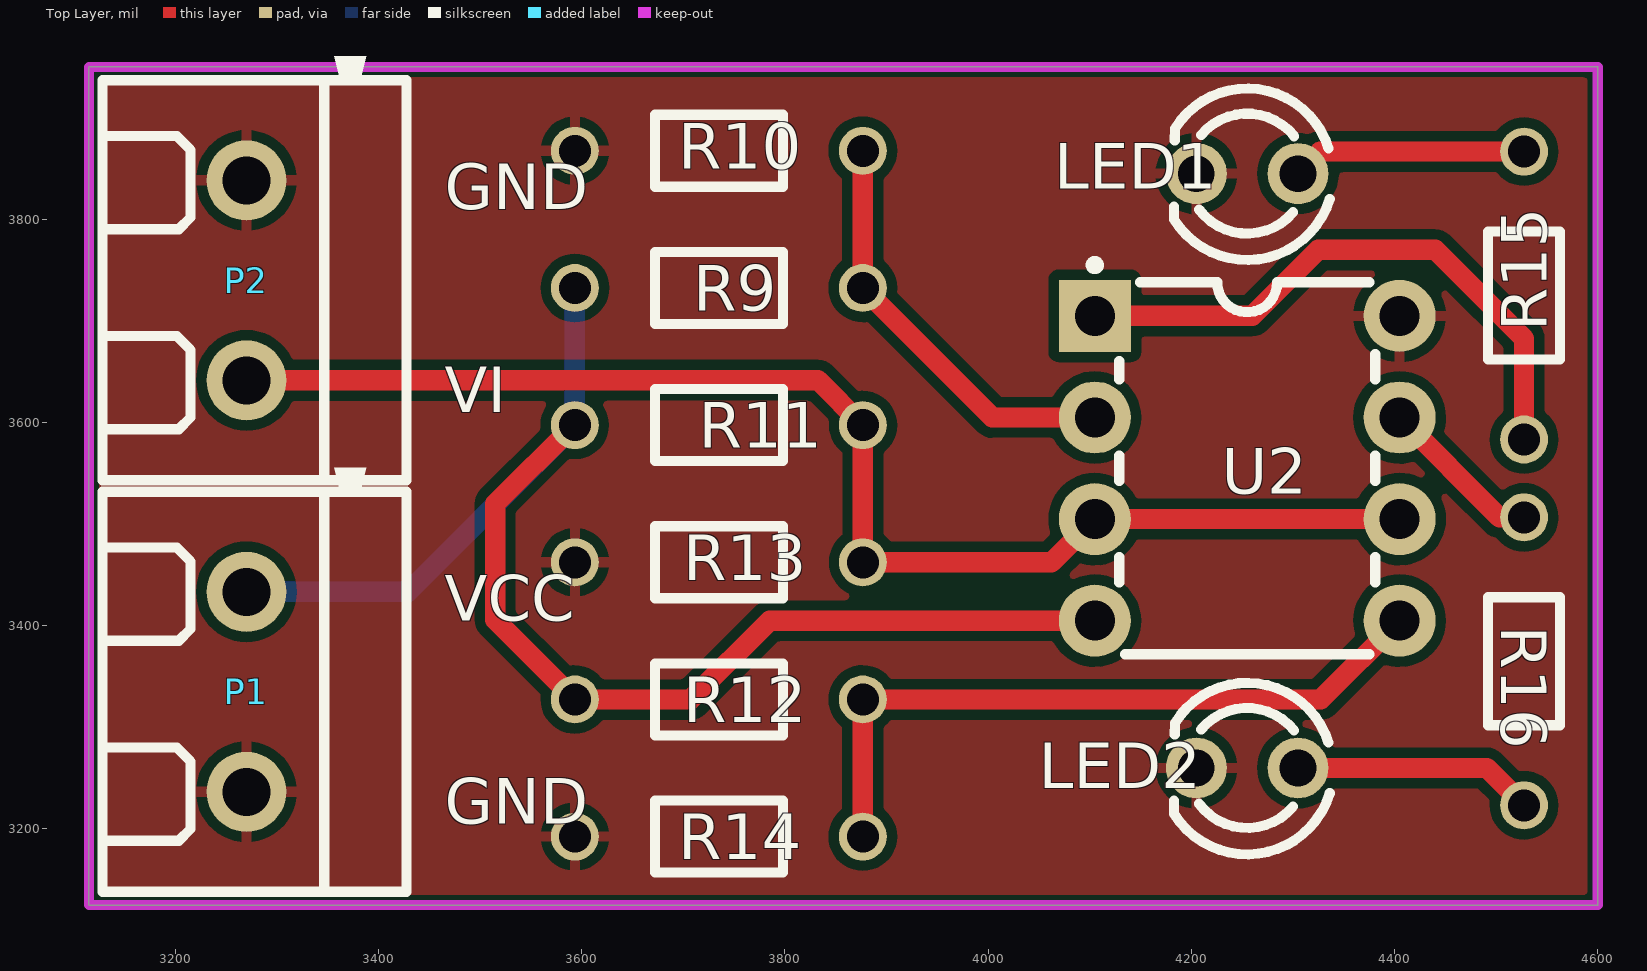
[diagram p0: Top Layer view]
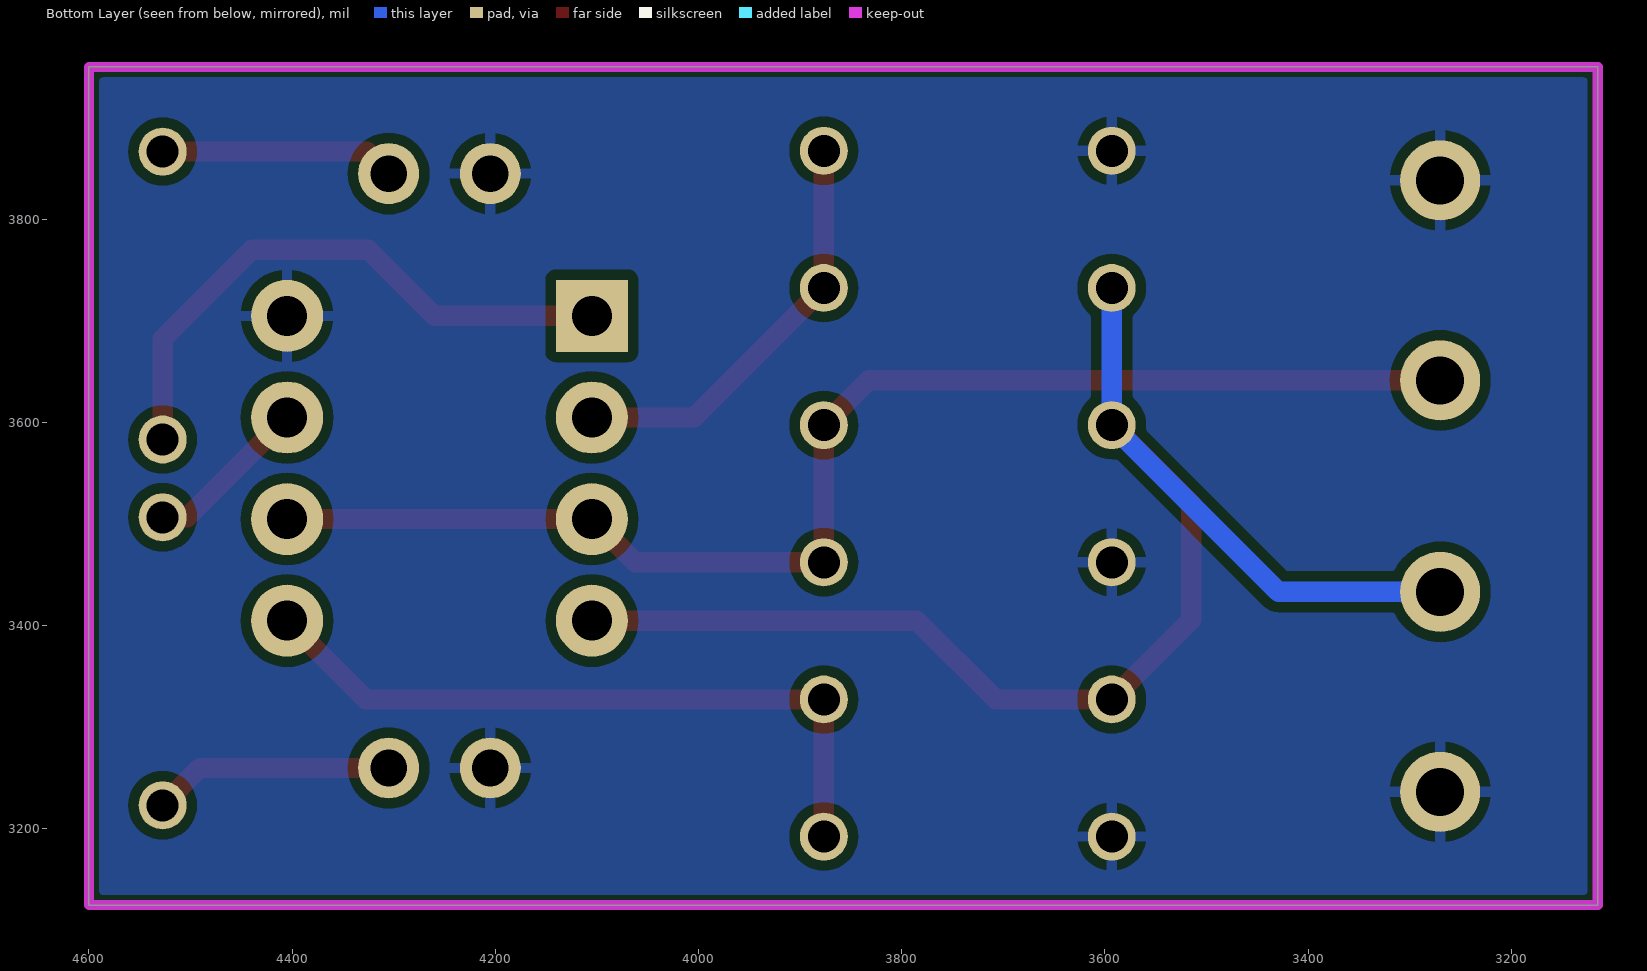
[diagram p1: Bottom Layer view, seen from below]
# Altium PCB MISC51032.pcbdoc
Units mil, origin at the board's own origin, x right, y up, seen from the top; angles counter-clockwise.
Board outline 1485 x 825 mil, 2 copper layers (Top Layer, Bottom Layer), stack 62.206 mil thick; 13 components, 9 nets, 32 pads, 0 vias.

## Layer stack, top to bottom
Top Solder Mask Layer: solder mask 0.394, Dk 3.3
Top Layer: signal copper 1.379
Dielectric1: surface 59.449, FR4, Dk 4.5
Bottom Layer: signal copper 1.378
Bottom Solder Mask Layer: solder mask 0.394, Dk 3.3

## Board outline
3115,3950 3115,3125 4600,3125 4600,3950

## Design rules (kind name [scope] priority, off if disabled: settings)
BoardOutlineClearance copperThickness2oz_1 [All] p2 off: genericclearance=7.99 ignorepadtopadclearanceinfootprint=FALSE except(0: Arc-SplitContinuation Track-SplitContinuation SMDPad-SplitContinuation THPad-SplitContinuation Via-SplitContinuation Fill-SplitContinuation Region-SplitContinuation Poly-SplitContinuation Text-SplitContinuation Hole-SplitContinuation; 5.98: Arc-CutoutEdge Track-CutoutEdge SMDPad-CutoutEdge THPad-CutoutEdge Via-CutoutEdge Text-CutoutEdge; 6.9: Hole-OutlineEdge Hole-CutoutEdge; 10: Poly-OutlineEdge Poly-CutoutEdge; 11.81: Arc-OutlineEdge Track-OutlineEdge SMDPad-OutlineEdge THPad-OutlineEdge Via-OutlineEdge Fill-OutlineEdge Region-OutlineEdge Text-OutlineEdge Fill-CutoutEdge Region-CutoutEdge)
BoardOutlineClearance Plane_innerPlane_1 [All] p4 off: genericclearance=4.02 ignorepadtopadclearanceinfootprint=FALSE except(0: Arc-SplitContinuation Track-SplitContinuation SMDPad-SplitContinuation THPad-SplitContinuation Via-SplitContinuation Fill-SplitContinuation Region-SplitContinuation Poly-SplitContinuation Text-SplitContinuation Hole-SplitContinuation; 5.98: Arc-CutoutEdge Track-CutoutEdge SMDPad-CutoutEdge THPad-CutoutEdge Via-CutoutEdge Text-CutoutEdge; 6.9: Hole-OutlineEdge Hole-CutoutEdge; 10: Poly-OutlineEdge Poly-CutoutEdge; 11.81: Arc-OutlineEdge Track-OutlineEdge SMDPad-OutlineEdge THPad-OutlineEdge Via-OutlineEdge Fill-OutlineEdge Region-OutlineEdge Text-OutlineEdge Fill-CutoutEdge Region-CutoutEdge)
BoardOutlineClearance Copper_copperRegion_1 [All] p6 off: genericclearance=4.02 ignorepadtopadclearanceinfootprint=FALSE except(0: Arc-SplitContinuation Track-SplitContinuation SMDPad-SplitContinuation THPad-SplitContinuation Via-SplitContinuation Fill-SplitContinuation Region-SplitContinuation Poly-SplitContinuation Text-SplitContinuation Hole-SplitContinuation; 5.98: Arc-CutoutEdge Track-CutoutEdge SMDPad-CutoutEdge THPad-CutoutEdge Via-CutoutEdge Text-CutoutEdge; 6.9: Hole-OutlineEdge Hole-CutoutEdge; 10: Poly-OutlineEdge Poly-CutoutEdge; 11.81: Arc-OutlineEdge Track-OutlineEdge SMDPad-OutlineEdge THPad-OutlineEdge Via-OutlineEdge Fill-OutlineEdge Region-OutlineEdge Text-OutlineEdge Fill-CutoutEdge Region-CutoutEdge)
BoardOutlineClearance copperThickness1oz_1 [All] p8: genericclearance=4.02 ignorepadtopadclearanceinfootprint=FALSE except(0: Arc-SplitContinuation Track-SplitContinuation SMDPad-SplitContinuation THPad-SplitContinuation Via-SplitContinuation Fill-SplitContinuation Region-SplitContinuation Poly-SplitContinuation Text-SplitContinuation Hole-SplitContinuation; 5.98: Arc-CutoutEdge Track-CutoutEdge SMDPad-CutoutEdge THPad-CutoutEdge Via-CutoutEdge Text-CutoutEdge; 6.9: Hole-OutlineEdge Hole-CutoutEdge; 10: Poly-OutlineEdge Poly-CutoutEdge; 11.81: Arc-OutlineEdge Track-OutlineEdge SMDPad-OutlineEdge THPad-OutlineEdge Via-OutlineEdge Fill-OutlineEdge Region-OutlineEdge Text-OutlineEdge Fill-CutoutEdge Region-CutoutEdge)
Clearance copperThickness2oz [All] p1 off: gap=7.99 ignorepadtopadclearanceinfootprint=FALSE except(5.98: SMDPad-Track SMDPad-SMDPad THPad-Track SMDPad-THPad THPad-THPad Track-Via SMDPad-Via THPad-Via Via-Via Fill-SMDPad Region-SMDPad Fill-THPad Region-THPad Fill-Via Region-Via Fill-Fill Fill-Region Region-Region Arc-Track Arc-SMDPad Arc-THPad Arc-Via Fill-Arc Region-Arc Arc-Arc Text-Track SMDPad-Text Text-THPad Text-Via Fill-Text Region-Text Arc-Text Text-Text; 6.9: Hole-Track Hole-SMDPad Hole-THPad Hole-Via Fill-Hole Region-Hole Hole-Arc Hole-Text; 10: Poly-Track Poly-SMDPad Poly-THPad Poly-Via Poly-Fill Poly-Region Poly-Poly Poly-Arc Poly-Text Poly-Hole; 11.81: Fill-Track Region-Track)
Clearance Plane_innerPlane [All] p3 off: gap=4.02 ignorepadtopadclearanceinfootprint=FALSE except(5.98: SMDPad-Track SMDPad-SMDPad THPad-Track SMDPad-THPad THPad-THPad Track-Via SMDPad-Via THPad-Via Via-Via Fill-SMDPad Region-SMDPad Fill-THPad Region-THPad Fill-Via Region-Via Fill-Fill Fill-Region Region-Region Arc-Track Arc-SMDPad Arc-THPad Arc-Via Fill-Arc Region-Arc Arc-Arc Text-Track SMDPad-Text Text-THPad Text-Via Fill-Text Region-Text Arc-Text Text-Text; 6.9: Hole-Track Hole-SMDPad Hole-THPad Hole-Via Fill-Hole Region-Hole Hole-Arc Hole-Text; 10: Poly-Track Poly-SMDPad Poly-THPad Poly-Via Poly-Fill Poly-Region Poly-Poly Poly-Arc Poly-Text Poly-Hole; 11.81: Fill-Track Region-Track)
Clearance Copper_copperRegion [All] p5 off: gap=4.02 ignorepadtopadclearanceinfootprint=FALSE except(5.98: SMDPad-Track SMDPad-SMDPad THPad-Track SMDPad-THPad THPad-THPad Track-Via SMDPad-Via THPad-Via Via-Via Fill-SMDPad Region-SMDPad Fill-THPad Region-THPad Fill-Via Region-Via Fill-Fill Fill-Region Region-Region Arc-Track Arc-SMDPad Arc-THPad Arc-Via Fill-Arc Region-Arc Arc-Arc Text-Track SMDPad-Text Text-THPad Text-Via Fill-Text Region-Text Arc-Text Text-Text; 6.9: Hole-Track Hole-SMDPad Hole-THPad Hole-Via Fill-Hole Region-Hole Hole-Arc Hole-Text; 10: Poly-Track Poly-SMDPad Poly-THPad Poly-Via Poly-Fill Poly-Region Poly-Poly Poly-Arc Poly-Text Poly-Hole; 11.81: Fill-Track Region-Track)
Clearance copperThickness1oz [All] p7: gap=4.02 ignorepadtopadclearanceinfootprint=FALSE except(5.98: SMDPad-Track SMDPad-SMDPad THPad-Track SMDPad-THPad THPad-THPad Track-Via SMDPad-Via THPad-Via Via-Via Fill-SMDPad Region-SMDPad Fill-THPad Region-THPad Fill-Via Region-Via Fill-Fill Fill-Region Region-Region Arc-Track Arc-SMDPad Arc-THPad Arc-Via Fill-Arc Region-Arc Arc-Arc Text-Track SMDPad-Text Text-THPad Text-Via Fill-Text Region-Text Arc-Text Text-Text; 6.9: Hole-Track Hole-SMDPad Hole-THPad Hole-Via Fill-Hole Region-Hole Hole-Arc Hole-Text; 10: Poly-Track Poly-SMDPad Poly-THPad Poly-Via Poly-Fill Poly-Region Poly-Poly Poly-Arc Poly-Text Poly-Hole; 11.81: Fill-Track Region-Track)
DiffPairsRouting differentialPair [All] p1: maxlimit=6 minlimit=6 mostfreqgap=6 toplayer_minwidth=5 toplayer_prefwidth=10 toplayer_maxwidth=100 toplayer_mingap=6 toplayer_prefgap=6 toplayer_maxgap=6 bottomlayer_minwidth=5 bottomlayer_prefwidth=10 bottomlayer_maxwidth=100 bottomlayer_mingap=6 bottomlayer_prefgap=6 bottomlayer_maxgap=6 maxuncoupledlength=10
HoleToHoleClearance otherClearance [All] p1: gap=11.81 allowstackedmicrovias=TRUE
Length netLength [All] p1: minlimit=0 maxlimit=0
PasteMaskExpansion pasteMaskExpansion [All] p1: expansion=0
PlaneConnect innerPlane [All] p1: planeconnectstyle=Relief reliefexpansion=20 reliefentries=4 reliefconductorwidth=10 reliefairgap=10
PolygonConnect copperRegion [All] p1: connectstyle=Relief reliefconductorwidth=10 reliefentries=4 polygonreliefangle="90 Angle" airgapwidth=10 via.connectstyle=Relief via.reliefconductorwidth=10 via.reliefentries=4 via.polygonreliefangle="90 Angle" via.airgapwidth=10
RoutingVias viaSize [All] p1: holewidth=12.01 width=24.02 viastyle="Through Hole" minholewidth=11.81 minwidth=19.68 maxholewidth=248.03 maxwidth=393.7
SolderMaskExpansion solderMaskExpansion [IsVia] p1: expansion=-1000 istentingtop=TRUE
SolderMaskExpansion solderMaskExpansion [All] p2: expansion=2 istentingtop=FALSE
Width copperThickness2oz_2 [All] p1 off: maxlimit=100 minlimit=8 preferedwidth=10
Width copperThickness1oz_2 [All] p2: maxlimit=100 minlimit=5 preferedwidth=10

## Components (designator, comment, footprint, x,y, rotation, side; value= is the part's Value field where it differs from the comment)
LED1 "" LED_TH-3mm 4255,3845 r180 top
LED2 "" LED_TH-3mm 4255,3260 r180 top
P1 "KF301-2P接线端子" CONN-TH_XY301V-A-5.0-2P 3270,3335 r90 top
P2 "KF301-2P接线端子" CONN-TH_XY301V-A-5.0-2P 3270,3740 r90 top
R9 "30K" Res_1/8W 3735,3730 r0 top
R10 "68K" Res_1/8W 3735,3865 r0 top
R11 "30K" Res_1/8W 3735,3599.95 r180 top
R12 "68K" Res_1/8W 3735,3325 r0 top
R13 "51K" Res_1/8W 3735,3460 r0 top
R14 "13K" Res_1/8W 3735,3190 r0 top
R15 "220" Res_1/8W 4529.95,3725 r90 top
R16 "220" Res_1/8W 4525,3365 r270 top
U2 "LM324AD" DIP-8_L9.3-W6.4-P2.54-LS7.6-BL 4255,3555 r270 top

## Footprints (in the part's own frame and the unit in brackets; to place one, negate y for a bottom-side part, rotate by r counter-clockwise, add the part's x,y. Pads: shape width x height; smd on the part's side, far side on the other; paste and mask are expansions set on the pad)
CONN-TH_XY301V-A-5.0-2P [mm]
  round 2 hole 1.2: 1(-2.5,0) 2(2.5,0)
  silkscreen extent -5,-4 5.6,3.6
DIP-8_L9.3-W6.4-P2.54-LS7.6-BL [mm]
  rect 1.8x1.8 hole 1: 1(-3.81,-3.81)
  round 1.8 hole 1: 2(-1.27,-3.81) 3(1.27,-3.81) 4(3.81,-3.81) 5(3.81,3.81) 6(1.27,3.81) 7(-1.27,3.81) 8(-3.81,3.81)
  silkscreen extent -5.18,-3.91 4.65,3.2
LED_TH-3mm [mil]
  round 60 hole 36 paste+0 mask+2: 1(-50,0) 2(50,0)
  silkscreen extent -81,-84 72,85
Res_1/8W [mil]
  round 47.2 hole 31.5 paste+0 mask+2: 1(-141.7,2.48) 2(141.7,2.48)
  silkscreen extent -63,-33 63,38

## Nets (pads, with @x,y where several pads share a name; then routed paths per layer and width w, separated by ;. In a path a pad name is that pad's centre, name@x,y a point inside that pad or via, vN(x,y) a via of type N, cw(c..) or ccw(c..) an arc to the next point about the centre after c; other vN are vias at no path point)
$1N193: R9.2 R10.2 U2.2 | length 416.1
  Top Layer w20: R10.2 R9.2 4004.18,3605 U2.2
$1N797: R12.2 R14.2 U2.5 | length 695.4
  Top Layer w20: R14.2 R12.2 4327.48,3327.48 U2.5
$1N964: LED1.1 R15.2 | length 231.5
  Top Layer w20: LED1.1 4326.7,3866.7 R15.2
$1N967: R15.1 U2.1 | length 584.9
  Top Layer w20: U2.1 4260,3705 4325,3770 4440,3770 4527.48,3682.52 R15.1
$1N1018: LED2.1 R16.2 | length 237.7
  Top Layer w20: LED2.1 4490.78,3260 R16.2
$1N1021: R16.1 U2.7 | length 163.2
  Top Layer w20: U2.7 4503.3,3506.7 R16.1
GND: LED1.2 LED2.2 P1.1 P2.2 R10.1 R13.1 R14.1 U2.8
VCC: P1.2 R9.1 R11.2 R12.1 U2.4 | length 1405.4
  Top Layer w20: R11.2 3592.48,3597.48 3515,3520 3515,3405.78 R12.1 3707.48,3327.48 3785,3405 U2.4
  Bottom Layer w20: P1.2 3429.25,3433.43 R11.2 R9.1
VI: P2.1 R11.1 R13.2 U2.3 U2.6 | length 1305.9
  Top Layer w20: P2.1 3832.6,3641.57 R11.1 R13.2 4062.48,3462.48 U2.3 U2.6

## Polygon pours and split planes (outlines as drawn)
GND on Bottom Layer (solid, remove dead copper, pour order 2): 3000,4030 3000,3040 4820,3040 4820,4030
GND on Top Layer (solid, remove dead copper, pour order 0): 3040,4020 3040,3000 4795,3000 4795,4020

## Keep-outs
Board Outline Layer:
  the board outline again, w10

## Silkscreen, mask and mechanical layers (free items; w line width, h text height)
Top Silkscreen Layer:
  text "GND" at 3465,3810 h45
  text "VI" at 3465,3610 h45
  text "VCC" at 3465,3405 h45
  text "GND" at 3465,3205 h45